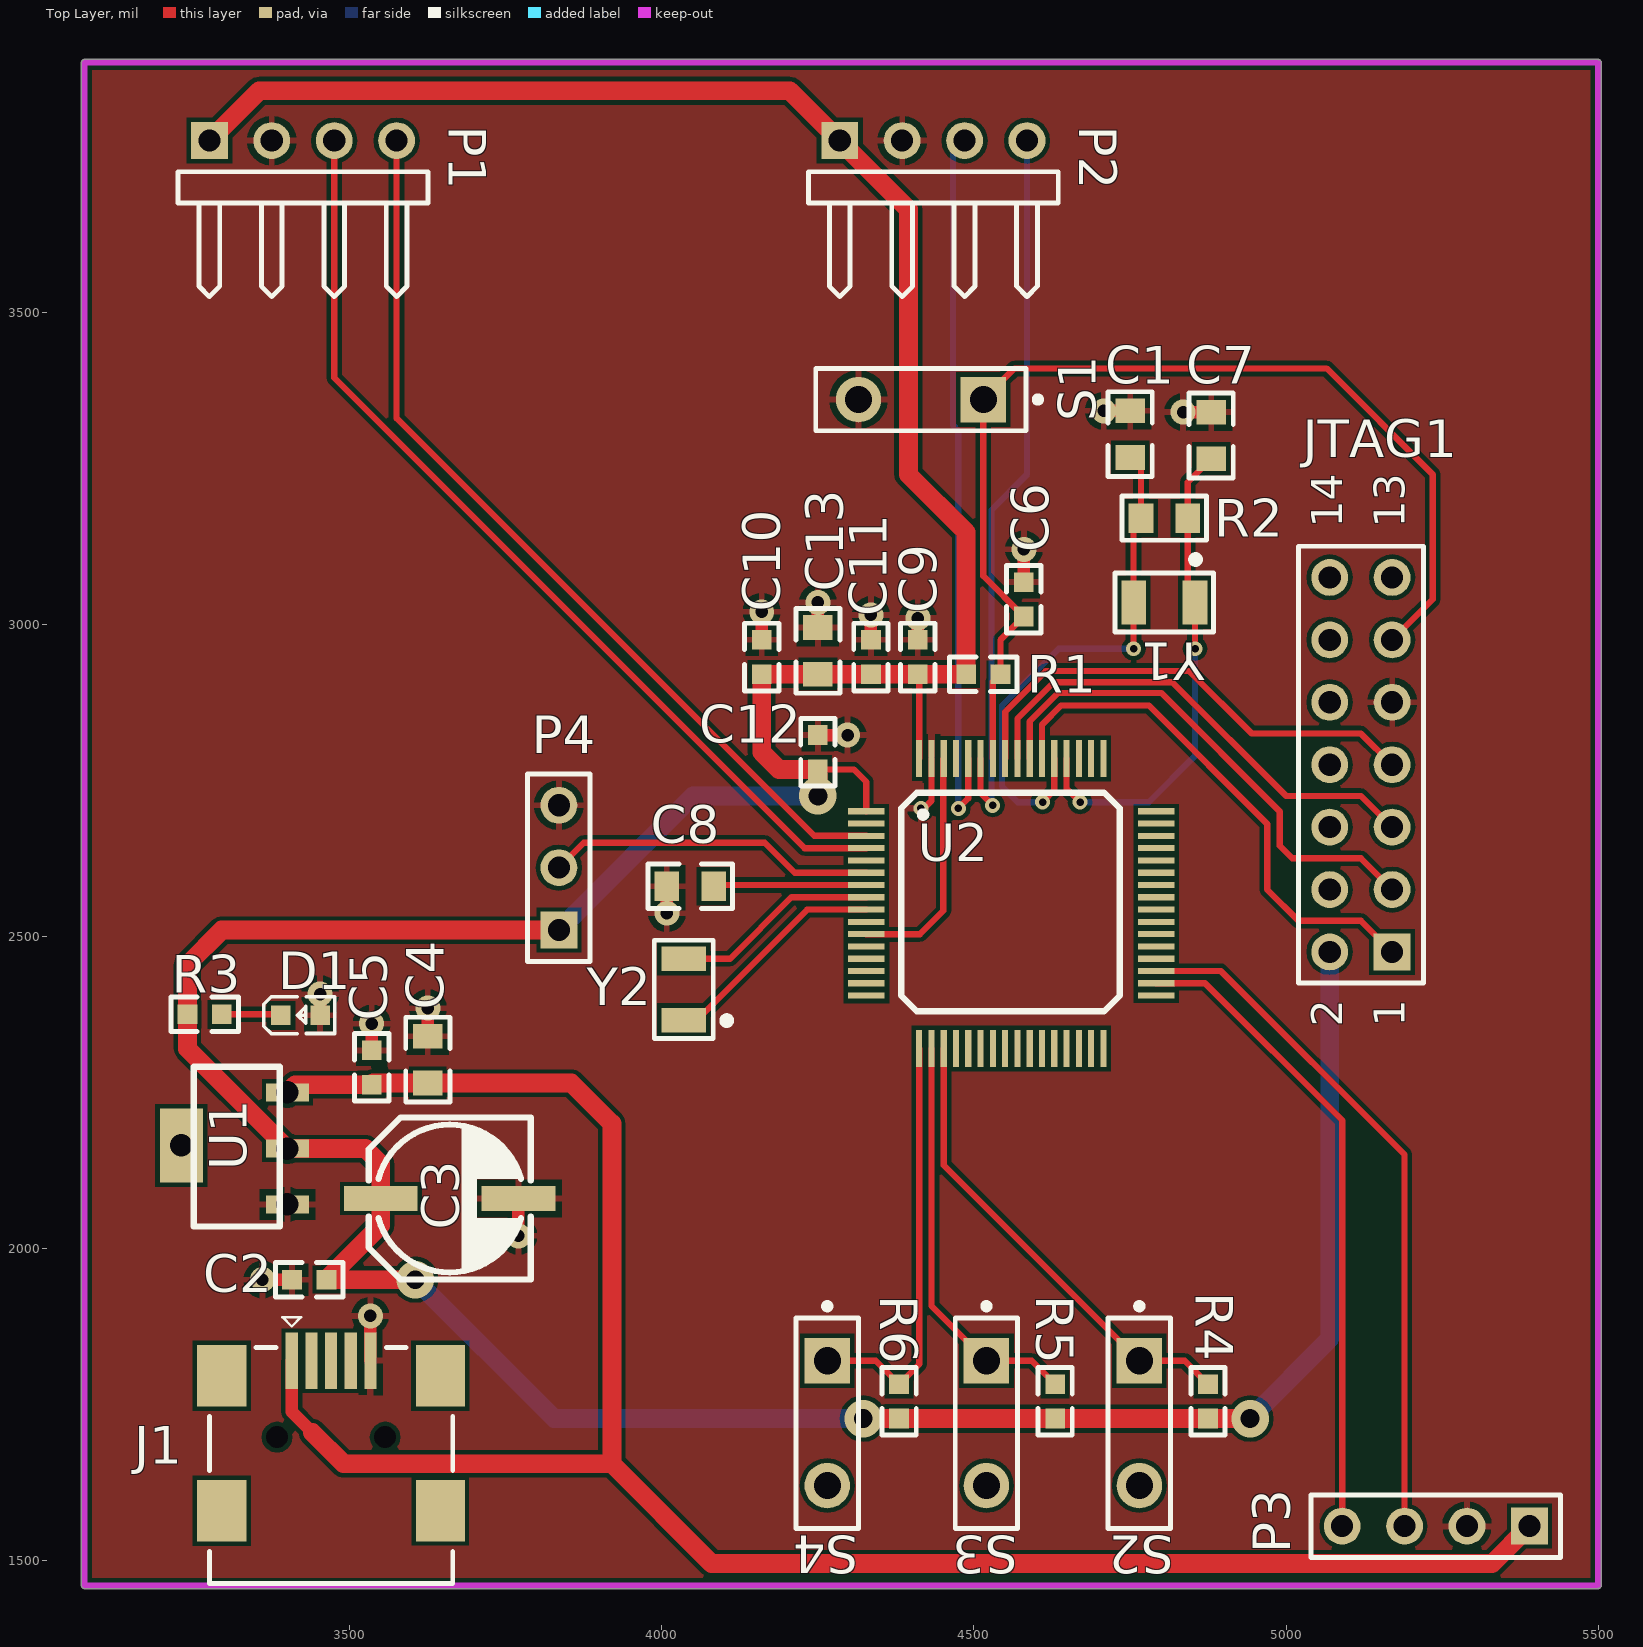
[diagram p0: Top Layer view]
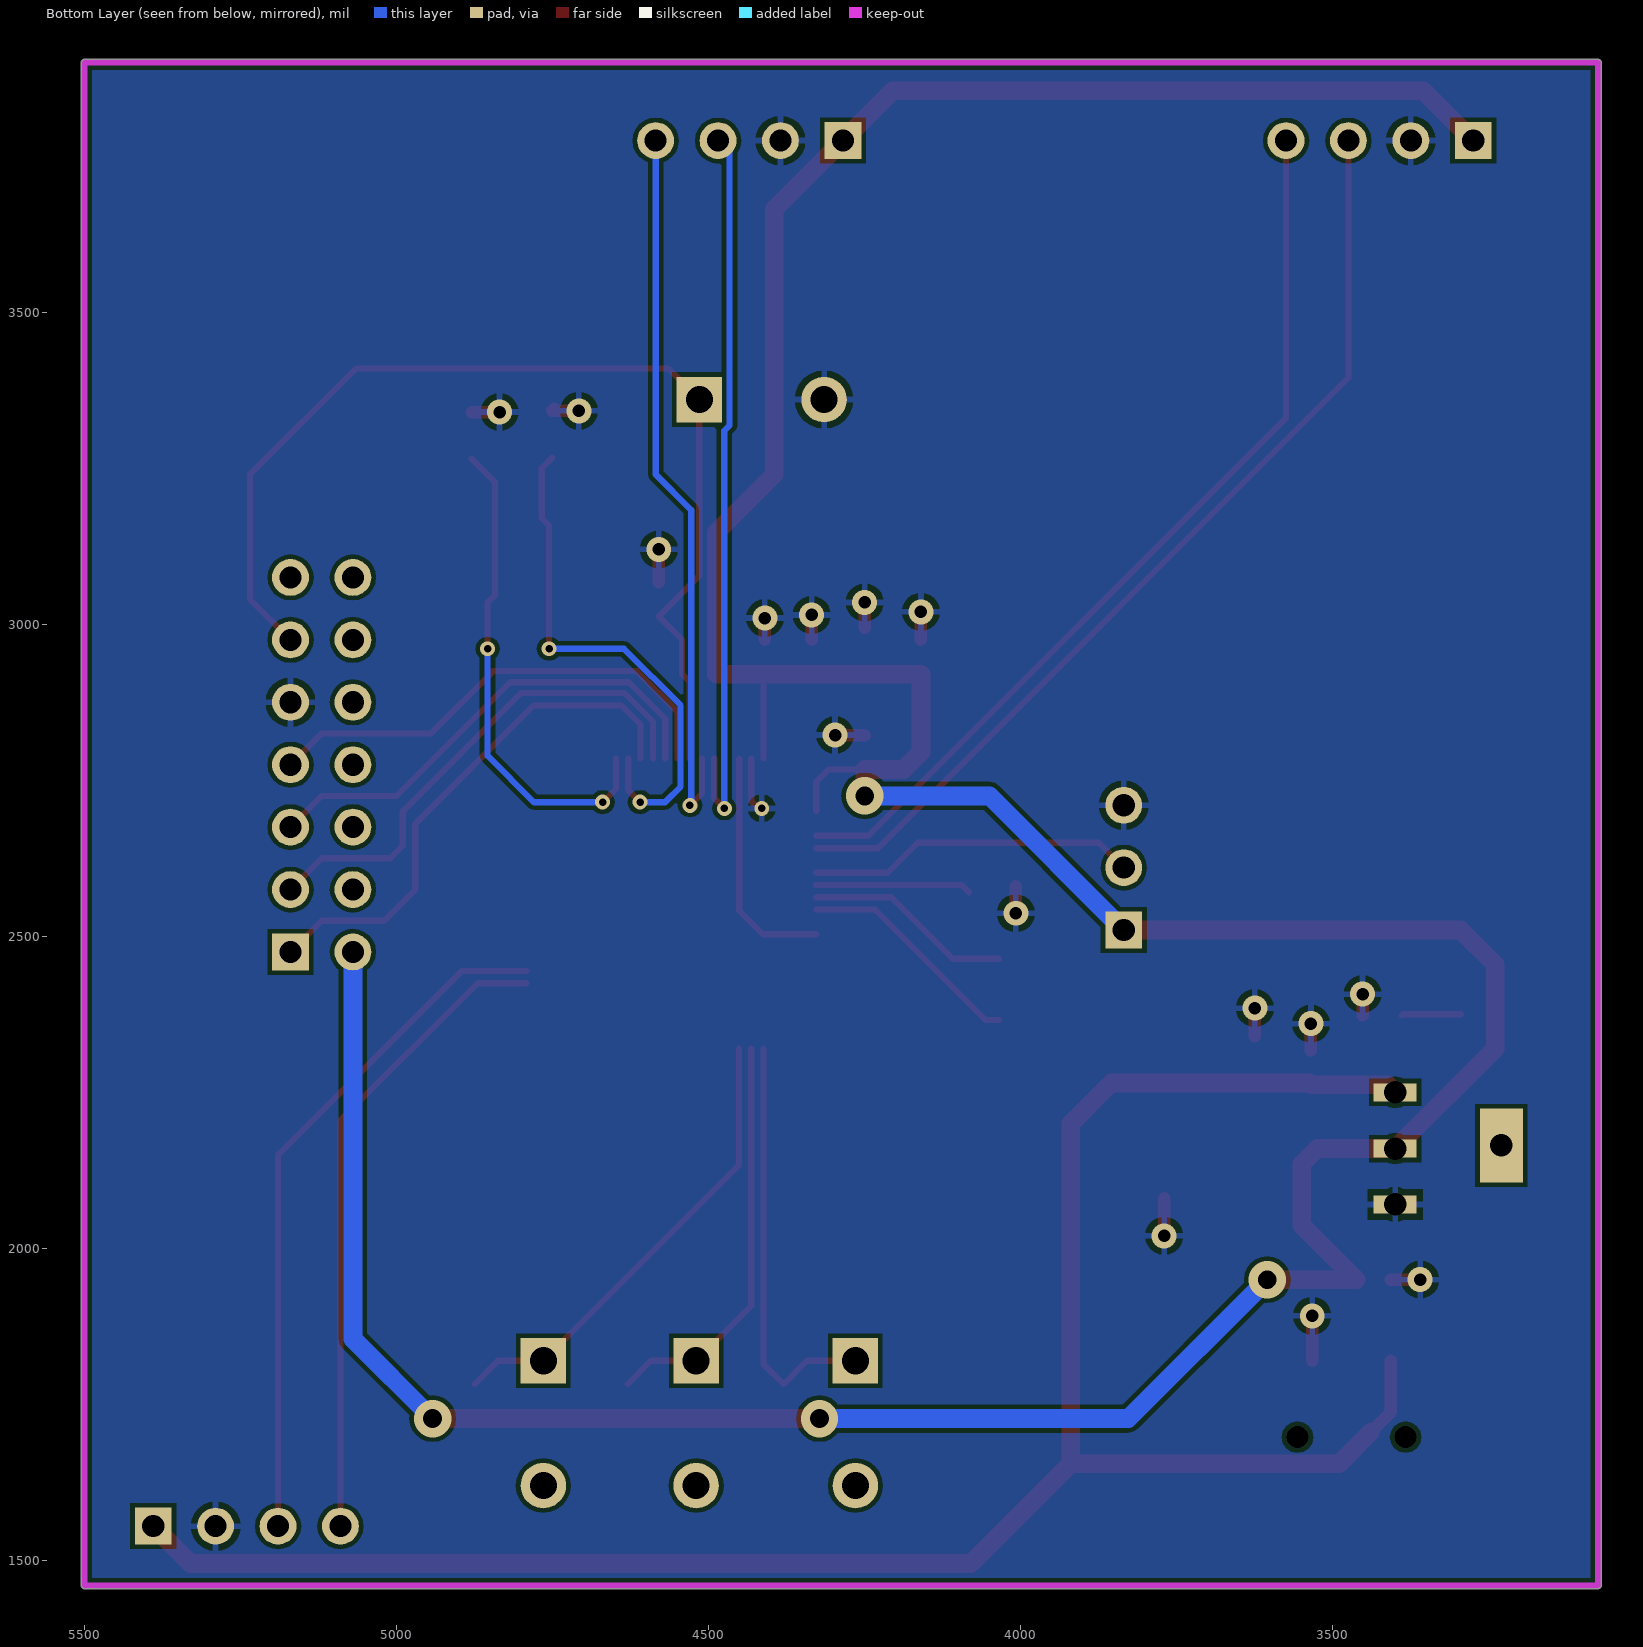
[diagram p1: Bottom Layer view, seen from below]
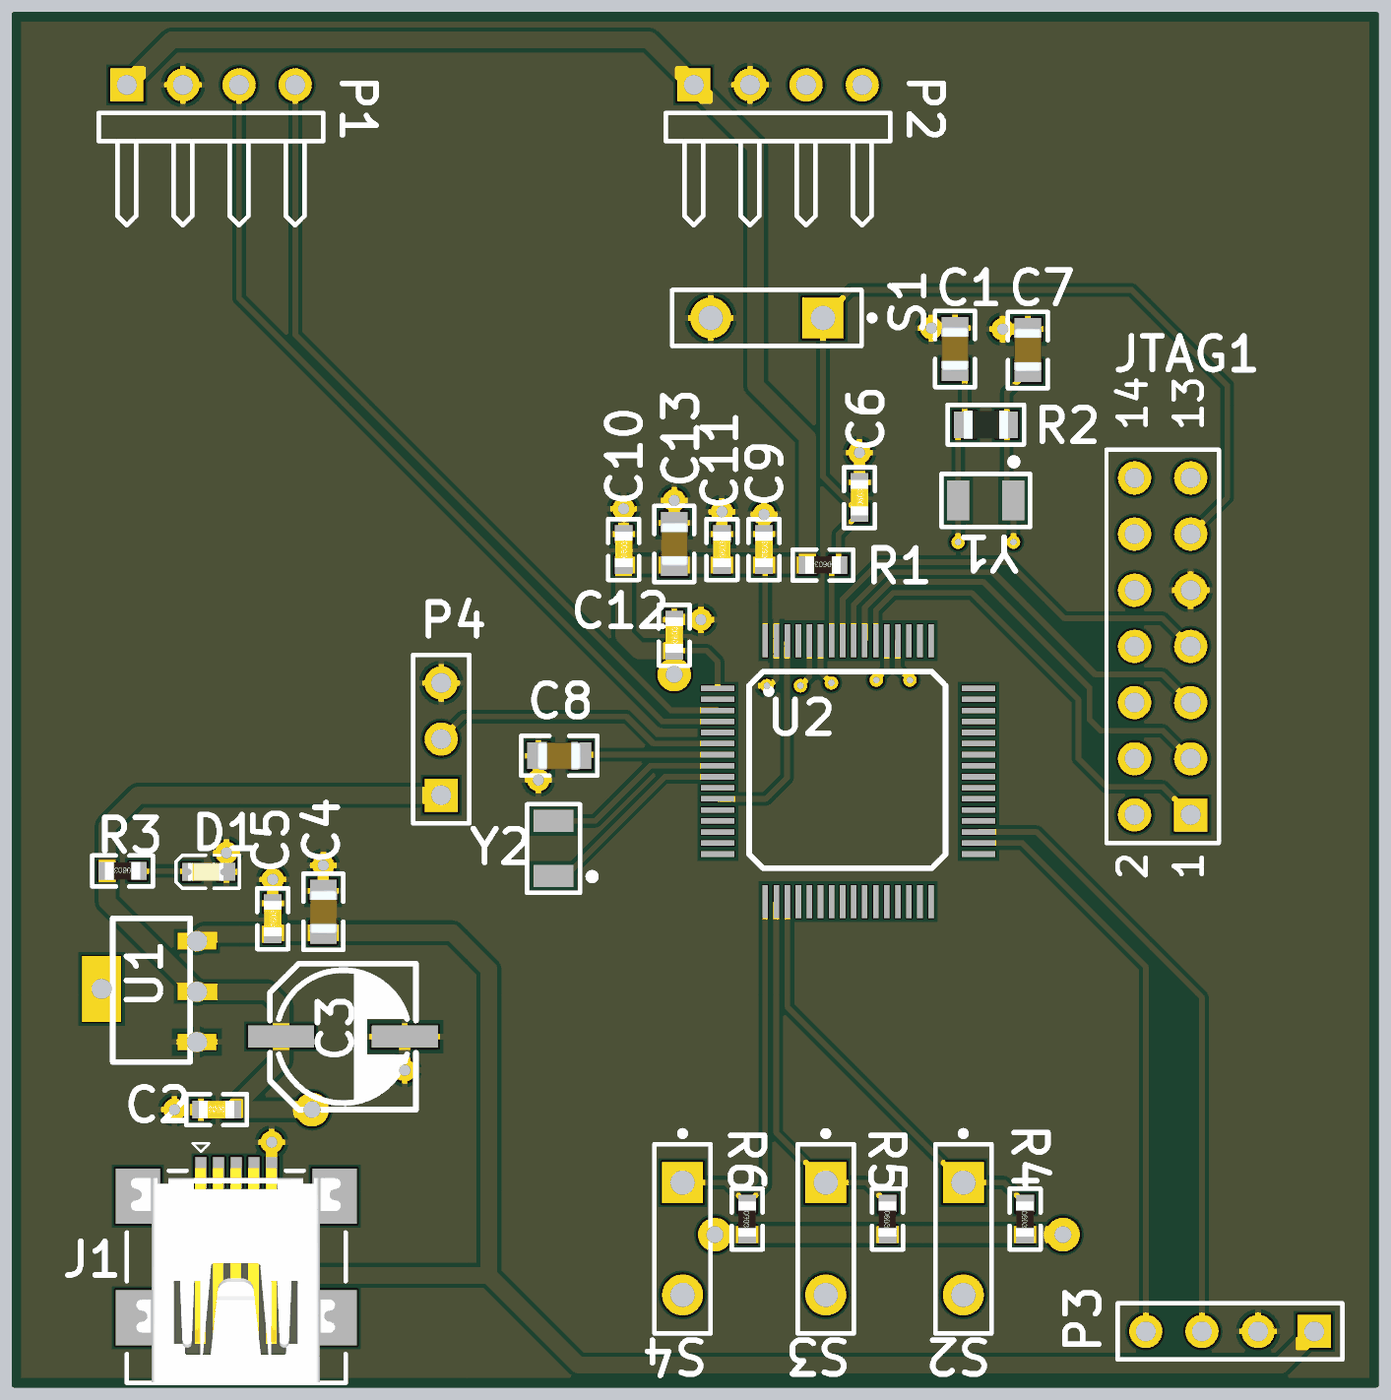
[diagram p2: 3D render of the assembled board from above, using the file's embedded part models]
# Altium PCB MISC82806.PcbDoc
Units mil, origin at the board's own origin, x right, y up, seen from the top; angles counter-clockwise.
Board outline 2435.03 x 2450.03 mil, 2 copper layers (Top Layer, Bottom Layer); 34 components, 63 nets, 160 pads, 26 vias.

## Layer stack, top to bottom (the 12.6 mil dielectric is the usual default, probably not edited)
Top Solder: solder mask 0.4, Solder Resist, Dk 3.5
Top Layer: signal copper 1.4
Dielectric 1: dielectric 12.6, FR-4, Dk 4.8
Bottom Layer: signal copper 1.4
Bottom Solder: solder mask 0.4, Solder Resist, Dk 3.5

## Board outline
3069.99,1460 ccw(c3075,1460) 3075,1454.98 5500,1454.98 ccw(c5500,1460) 5505.02,1460 5505.02,3900 ccw(c5500,3900) 5500,3905.01 3075,3905.01 ccw(c3075,3900) 3069.99,3900

## Design rules (kind name [scope] priority, off if disabled: settings)
Clearance [All] p1: gap=7
MinimumSolderMaskSliver [All] p1: minsoldermaskwidth=0
PolygonConnect [All] p1: connectstyle=Relief reliefconductorwidth=10 reliefentries=4 polygonreliefangle="90 Angle" airgapwidth=10
RoutingVias [All] p1: holewidth=28 width=50 viastyle="Through Hole" minholewidth=28 minwidth=50 maxholewidth=28 maxwidth=50
SilkToSilkClearance [All] p1: silktosilkclearance=0
SilkToSolderMaskClearance [IsPad] p1: minsilkscreentomaskgap=0 clearancetoexposedcopper=TRUE
SolderMaskExpansion [All] p1: expansion=4
Width [All] p1: maxlimit=30 minlimit=10 preferedwidth=10
27 further rules are at their usual default settings.

## Components (designator, comment, footprint, x,y, rotation, side; value= is the part's Value field where it differs from the comment)
C1 "S0805-20P" 0805C 4750,3305 r270 top
C2 "104" 0603C 3435,1950 r180 top
C3 "10uF" 贴片电容 3660,2080 r270 top
C4 "10uF" 0805C 3625.28,2302.01 r90 top
C5 "104" 0603C 3535,2290 r90 top
C6 "104" 0603C 4580,3040 r90 top
C7 "S0805-20P" 0805C 4879.72,3302.99 r270 top
C8 "S0805-20P" 0805C 4045,2580 r0 top
C9 "104" 0603C 4410,2947.56 r90 top
C10 "104" 0603C 4160,2947.56 r90 top
C11 "104" 0603C 4335,2947.56 r90 top
C12 "104" 0603C 4250,2795 r90 top
C13 "106" 0805C 4250.28,2957.01 r90 top
D1 "LED0" LED0603-RD 3420.93,2373.5 r0 top
J1 "Mini-USB" USB-MINI-A 3407.01,1820 r0 top
JTAG1 "DIP14" HDR2X7 5170,2475 r90 top
P1 "OLED" HDR1X4H 3275,3775 r0 top
P2 "BMP108" HDR1X4H 4285,3775 r0 top
P3 "Bluetooth module" HDR1X4 5390,1555 r180 top
P4 "Buzzer" HDR1X3 3835,2510 r90 top
R1 "10K" 0603R 4515,2920 r180 top
R2 "RC-1M" 0805R 4805,3170 r180 top
R3 "510R" 0603R 3267.44,2375 r180 top
R4 "10K" 0603R 4875,1755 r270 top
R5 "10K" 0603R 4630,1755 r270 top
R6 "10K" 0603R 4380,1755 r270 top
S1 "SW-SPST" SPST-2 4415,3360 r180 top
S2 "SW-PB" SPST-2 4765,1720 r270 top
S3 "SW-PB" SPST-2 4520,1720 r270 top
S4 "SW-PB" SPST-2 4265,1720 r270 top
U1 "AMS1117-3.3" AMS1117-3.3 3289.72,2052.95 r90 top
U2 "MSP430F149" MSP430F149 4559.84,2552.72 r0 top
Y1 "8M" XTAL-SMD-NX3215SA-32.768K-STD-MUS-2 4805,3035 r180 top
Y2 "32768" XTAL-SMD-NX3215SA-32.768K-STD-MUS-2 4035,2415 r90 top

## Footprints (in the part's own frame and the unit in brackets; to place one, negate y for a bottom-side part, rotate by r counter-clockwise, add the part's x,y. Pads: shape width x height; smd on the part's side, far side on the other; paste and mask are expansions set on the pad)
0603C [mm]
  rect 0.8x0.8 smd: 1(-0.7,0) 2(0.7,0)
  silkscreen extent -1.38,-0.7 1.38,0.7, body extent -0.8,-0.4 0.8,0.4, height 0.8
0603R [mm]
  rect 0.8x0.8 smd: 1(-0.7,0) 2(0.7,0)
  silkscreen extent -1.38,-0.7 1.38,0.7, body extent -0.8,-0.41 0.8,0.39, height 0.8
0805C [mm]
  rect 1x1.2 smd: 1(-0.94,0.007) 2(0.96,0.007)
  silkscreen extent -1.72,-0.89 1.74,0.91, body extent -1,-0.63 1,0.63, height 1.45
0805R [mm]
  rect 1x1.2 smd: 1(-0.95,0) 2(0.95,0)
  silkscreen extent -1.73,-0.9 1.73,0.9, body extent -1,-0.64 1,0.64, height 0.65
AMS1117-3.3 [mm]
  rect 0.74x1.75 hole 0.914 paste+0 mask+0.051: 1(0.444,-2.801) 2(2.719,-2.801) 3(5.005,-2.801)
  rect 3x1.75 hole 0.914 paste+0 mask+0.051: 4(2.846,1.517)
  silkscreen extent -0.46,-2.49 6.04,1.01
HDR1X3 [mm] "Connector; Header; 3 Position"
  rect 1.5x1.5 hole 0.9: 1(0,0)
  round 1.5 hole 0.9: 2(2.54,0) 3(5.08,0)
  silkscreen extent -1.27,-1.27 6.35,1.27
HDR1X4 [mm] "Connector; Header; 4 Position"
  rect 1.5x1.5 hole 0.9: 1(0,0)
  round 1.5 hole 0.9: 2(2.54,0) 3(5.08,0) 4(7.62,0)
  silkscreen extent -1.27,-1.27 8.89,1.27
HDR1X4H [mm] "Connector; Header; 4 Position; Right Angle"
  rect 1.5x1.5 hole 0.9: 1(0,0)
  round 1.5 hole 0.9: 2(2.54,0) 3(5.08,0) 4(7.62,0)
  silkscreen extent -1.27,-6.35 8.89,-1.27
HDR2X7 [mm] "Connector; Header; 7x2 Position"
  rect 1.5x1.5 hole 0.9: 1(0,0)
  round 1.5 hole 0.9: 2(0,2.54) 3(2.54,0) 4(2.54,2.54) 5(5.08,0) 6(5.08,2.54) 7(7.62,0) 8(7.62,2.54) 9(10.16,0) 10(10.16,2.54) 11(12.7,0) 12(12.7,2.54) 13(15.24,0) 14(15.24,2.54)
  silkscreen extent -1.27,-1.27 16.51,3.81
LED0603-RD [mm]
  rect 0.8x0.8 smd: 1(-0.8,-0.003) 2(0.8,0.003)
  silkscreen extent -1.49,-0.75 1.39,0.76, body extent -0.93,-0.4 0.67,0.4, height 0.55
MSP430F149 [mm]
  rect 1.5x0.25 smd paste+0 mask+0.051: 1(-5.9,3.75) 2(-5.9,3.25) 3(-5.9,2.75) 4(-5.9,2.25) 5(-5.9,1.75) 6(-5.9,1.25) 7(-5.9,0.75) 8(-5.9,0.25) 9(-5.9,-0.25) 10(-5.9,-0.75) 11(-5.9,-1.25) 12(-5.9,-1.75) 13(-5.9,-2.25) 14(-5.9,-2.75) 15(-5.9,-3.25) 16(-5.9,-3.75) 33(5.9,-3.75) 34(5.9,-3.25) 35(5.9,-2.75) 36(5.9,-2.25) 37(5.9,-1.75) 38(5.9,-1.25) 39(5.9,-0.75) 40(5.9,-0.25) 41(5.9,0.25) 42(5.9,0.75) 43(5.9,1.25) 44(5.9,1.75) 45(5.9,2.25) 46(5.9,2.75) 47(5.9,3.25) 48(5.9,3.75)
  rect 0.25x1.5 smd paste+0 mask+0.051: 17(-3.75,-5.9) 18(-3.25,-5.9) 19(-2.75,-5.9) 20(-2.25,-5.9) 21(-1.75,-5.9) 22(-1.25,-5.9) 23(-0.75,-5.9) 24(-0.25,-5.9) 25(0.25,-5.9) 26(0.75,-5.9) 27(1.25,-5.9) 28(1.75,-5.9) 29(2.25,-5.9) 30(2.75,-5.9) 31(3.25,-5.9) 32(3.75,-5.9) 49(3.75,5.9) 50(3.25,5.9) 51(2.75,5.9) 52(2.25,5.9) 53(1.75,5.9) 54(1.25,5.9) 55(0.75,5.9) 56(0.25,5.9) 57(-0.25,5.9) 58(-0.75,5.9) 59(-1.25,5.9) 60(-1.75,5.9) 61(-2.25,5.9) 62(-2.75,5.9) 63(-3.25,5.9) 64(-3.75,5.9)
  silkscreen extent -4.48,-4.38 4.41,4.51
SPST-2 [mm] "Switch; 2 Leads"
  rect 1.85x1.85 hole 1.1: 1(-2.54,0)
  round 1.85 hole 1.1: 2(2.54,0)
  silkscreen extent -4.89,-1.27 4.28,1.27
USB-MINI-A [mm]
  rect 2x2.5 smd: 0(-2.85,-6.108) 0(-2.85,-0.608) 0(6.05,-6.108) 0(6.05,-0.608)
  rect 0.5x2.3 smd: 1(0,0) 2(0.8,0) 3(1.6,0) 4(2.4,0) 5(3.2,0)
  round 0.6 hole 0.9 unplated: MH1(3.8,-3.108) MH2(-0.6,-3.108)
  silkscreen extent -3.35,-9.06 6.55,1.78, body extent -3.17,-9.04 6.33,0.66, height 3.95
XTAL-SMD-NX3215SA-32.768K-STD-MUS-2 [mm] "Crystal; 3.2mm W X 1.5mm L X 0.9mm H body"
  rect 1x1.8 smd paste+0 mask+0: 1(-1.25,0) 2(1.25,0)
  silkscreen extent -2,-1.9 2,1.2, body extent -1.6,-0.75 1.6,0.75, height 0.9
贴片电容 [mm]
  rect 1x3 smd paste+0 mask+0.102: 1(0,-2.8) 2(0,2.8)
  silkscreen extent -3.3,-3.3 3.3,3.3

## Part data
C1 C2 C7 C8: library part Cap, "Capacitor"
C3: library part "CAPACITOR POL", "Capacitor"
C4: library part ELECTRO2
C5: library part CAP, "Capacitor"
C6 C9 C10 C11 C12 C13: library part CAP1, "Capacitor"
D1: "Typical INFRARED GaAs LED"
J1: library part "Header 5", "Header, 5-Pin"
JTAG1: "Connectors"
P1 P2: library part "Header 4H", "Header, 4-Pin, Right Angle"
P3: library part "Header 4", "Header, 4-Pin"
P4: library part "Header 3", "Header, 3-Pin"
R1 R3 R4 R5 R6: library part R
R2: library part Res2, "Resistor"
S1: "Single-Pole, Single-Throw Switch"
S2 S3 S4: "Switch"
U1: library part LT1085CM-3.3
U2: "MCU"
Y1 Y2: library part XTAL, "Crystal Oscillator"

## Via types
v1: diameter 40, hole 20, Top Layer to Bottom Layer, 15 vias
v2: diameter 24, hole 12, Top Layer to Bottom Layer, 7 vias
v3: diameter 60, hole 30, Top Layer to Bottom Layer, 4 vias

## Nets (pads, with @x,y where several pads share a name; then routed paths per layer and width w, separated by ;. In a path a pad name is that pad's centre, name@x,y a point inside that pad or via, vN(x,y) a via of type N, cw(c..) or ccw(c..) an arc to the next point about the centre after c; other vN are vias at no path point)
3V3: C2.1 C3.1 C9.1 C10.1 C11.1 C12.1 C13.1 JTAG1.2 P1.1 P2.1 P4.1 R1.2 R3.2 R4.2 R5.2 R6.2 U1.2 U2.1 U2.64 | length 7117.3
  Top Layer w10: C12.1 4307.56,2767.44 4327.55,2747.45 U2.1 ; C9.1 4412.2,2917.8 U2.64
  Top Layer w30: P1.1 3355,3855 4205,3855 P2.1 4395,3665 4395,3240 4487.44,3147.56 R1.2 C9.1 C11.1 C13.1 C10.1 4160,2795 4187.56,2767.44 C12.1 v3(4250,2725) ; v3(3605,1950) C2.1 3549.76,2037.2 C3.1 3549.76,2135.24 3525,2160 U1.2 3239.88,2320.12 R3.2 3239.88,2454.88 3295,2510 P4.1 ; v3(4322.44,1727.44) R6.2 R5.2 R4.2 v3(4942.44,1727.44)
  Bottom Layer w30: v3(3605,1950) 3827.56,1727.44 v3(4322.44,1727.44) ; P4.1 4050,2725 v3(4250,2725) ; v3(4942.44,1727.44) 5070,1855 JTAG1.2
5V: C4.1 C5.1 J1.1 P3.1 U1.3 | length 3288.6
  Top Layer w20: J1.1 3407.01,1737.99 3440,1705
  Top Layer w30: U1.3 3412.44,2262.44 C5.1 3537.56,2265 C4.1 3855,2265 3920,2200 3920,1655 ; 3440,1705 3490,1655 3920,1655 ; P3.1 5330,1495 4080,1495 3920,1655
GND: C1.1 C2.2 C3.2 C4.2 C5.2 C6.2 C7.1 C8.1 C9.2 C10.2 C11.2 C12.2 C13.2 D1.2 J1.5 JTAG1.9 P1.2 P2.2 P3.2 P4.3 S1.2 U1.1 U2.63 | length 785.2
  Top Layer w10: v2(4415,2705) 4420,2705 4431.89,2716.89 U2.63
  Top Layer w20: v1(3360,1950) C2.2 ; D1.2 v1(3452.4,2407.4) ; J1.5 v1(3532.99,1892.01) ; C5.2 v1(3535,2360) ; C4.2 v1(3625,2385) ; v1(3770.24,2020.24) C3.2 ; v1(4007.99,2537.01) C8.1 ; C10.2 v1(4160,3020) ; C12.2 v1(4297.56,2822.56) ; C13.2 v1(4250,3035) ; C11.2 v1(4335,3015) ; C9.2 v1(4410,3010) ; C6.2 v1(4580,3120) ; v1(4707.99,3342.01) C1.1 C1.1@4747.28,3345 ; v1(4835,3340) C7.1
GNDA: U2.11 U2.62 | length 383.2
  Top Layer w10: U2.11 4413.51,2503.51 4451,2541 4451,2784.43 U2.62
NetC8_2: C8.2 U2.7 | length 249.7
  Top Layer w10: C8.2@4082.8,2570.28 4094.77,2582.25 U2.7
NetD1_1: D1.1 R3.1 | length 95.1
  Top Layer w10: R3.1 3387.82,2375 D1.1
NETLABEL41: U2.49
NetU2_8: U2.8 Y2.2 | length 333.3
  Top Layer w10: Y2.2 4109.21,2464.21 4207.56,2562.56 U2.8
NetU2_9: U2.9 Y2.1 | length 365.9
  Top Layer w10: Y2.1 4055.79,2365.79 4232.88,2542.88 U2.9
P1.0: U2.12
P1.1: U2.13
P1.2: U2.14
P1.3: U2.15
P1.4: U2.16
P1.5: R6.1 S4.1 U2.17 | length 681.7
  Top Layer w10: S4.1 4342.56,1820 R6.1 4412.2,1814.76 U2.17
P1.6: R5.1 S3.1 U2.18 | length 662.4
  Top Layer w10: U2.18 4431.89,1908.11 S3.1 4592.56,1820 R5.1
P1.7: R4.1 S2.1 U2.19 | length 755.8
  Top Layer w10: U2.19 4451.57,2133.43 S2.1 4837.56,1820 R4.1
P2.0: U2.20
P2.1: U2.21
P2.2: U2.22
P2.3: U2.23
P2.4: U2.24
P2.5: U2.25
P2.6: U2.26
P2.7: U2.27
P3.0: U2.28
P3.1: U2.29
P3.2: U2.30
P3.3: U2.31
P3.4: U2.32
P3.5: U2.33
P3.6: P3.4 U2.34 | length 1038.9
  Top Layer w10: U2.34 4870.24,2424.76 5090,2205 P3.4
P3.7: P3.3 U2.35 | length 1114.8
  Top Layer w10: U2.35 4895.55,2444.45 5190,2150 P3.3
P4.0: U2.36
P4.1: U2.37
P4.2: U2.38
P4.3: U2.39
P4.4: U2.40
P4.5: U2.41
P4.6: U2.42
P4.7: U2.43
P5.0: U2.44
P5.1: U2.45
P5.2: U2.46
P5.3: U2.47
P5.4: U2.48
P5.7: U2.51
P6.0: P2.4 U2.59 | length 1172.5
  Top Layer w10: U2.59 4510.63,2729.37 v2(4530,2710)
  Bottom Layer w10: v2(4530,2710) 4528,2712 4528,3183 4585,3240 P2.4
P6.1: P2.3 U2.60 | length 1167.7
  Top Layer w10: v2(4475,2705) 4490.94,2720.94 U2.60
  Bottom Layer w10: v2(4475,2705) 4475,3310.19 4466.58,3318.61 4466.58,3756.58 P2.3
P6.2: U2.61
P6.3: U2.2
P6.4: P1.4 U2.3 | length 1474.7
  Top Layer w10: P1.4 3575,3330 4244.01,2660.99 U2.3
P6.5: P1.3 U2.4 | length 1544.7
  Top Layer w10: P1.3 3475,3395 4228.7,2641.3 U2.4
P6.6: U2.5
P6.7: P4.2 U2.6 | length 529
  Top Layer w10: P4.2 3875,2650 4165,2650 4213.07,2601.93 U2.6
RESET: C6.1 JTAG1.11 R1.1 S1.1 U2.58 | length 1725.6
  Top Layer w10: U2.58 4530.31,2907.75 R1.1 4542.56,2975 C6.1 4515,3077.44 S1.1 4565,3410 5065,3410 5235,3240 5235,3040 JTAG1.11
TCK: JTAG1.7 U2.57 | length 784.1
  Top Layer w10: U2.57 4550,2860 4615,2925 4845,2925 4945,2825 5120,2825 JTAG1.7
TDI: JTAG1.3 U2.55 | length 821.6
  Top Layer w10: U2.55 4589.37,2844.37 4635,2890 4800,2890 4990,2700 4990,2645 5010,2625 5120,2625 JTAG1.3
TDO: JTAG1.1 U2.54 | length 852.9
  Top Layer w10: U2.54 4609.05,2839.05 4640,2870 4780,2870 4970,2680 4970,2575 5020,2525 5120,2525 JTAG1.1
TMS: JTAG1.5 U2.56 | length 784.3
  Top Layer w10: U2.56 4569.68,2848.72 4627.96,2907 4818,2907 5000,2725 5120,2725 JTAG1.5
VEREF+: U2.10
XT2_IN: C1.2 R2.2 U2.53 Y1.2 | length 850
  Top Layer w10: v2(4610,2715) 4628.74,2733.74 U2.53 ; C1.2 4767.6,3249.88 R2.2 4755.79,3158.19 Y1.2 v2(4755.79,2960.79)
  Bottom Layer w10: v2(4610,2715) 4570,2715 4545,2740 4545,2870 4635.79,2960.79 v2(4755.79,2960.79)
XT2_OUT: C7.2 R2.1 U2.52 Y1.1 | length 790.3
  Top Layer w10: U2.52 4648.42,2736.58 v2(4670,2715) ; v2(4854.21,2960.79) Y1.1 4842.4,3046.81 R2.1 4842.4,3227.6 C7.2
  Bottom Layer w10: v2(4670,2715) 4780,2715 4854.21,2789.21 v2(4854.21,2960.79)
pads on no net: J1.0 J1.2 J1.3 J1.4 J1.MH1 J1.MH2 JTAG1.4 JTAG1.6 JTAG1.8 JTAG1.10 JTAG1.12 JTAG1.13 JTAG1.14 S2.2 S3.2 S4.2 U1.4 U2.50

## Polygon pours and split planes (outlines as drawn)
GND on Top Layer "G" (solid, remove dead copper, pour order 0): 2245,4060 2270,4085 5880,4085 5880,1645 5585,1350 5560,1325 2755,1325
GND on Bottom Layer "G" (solid, remove dead copper, pour order 2): 2970,3975 5525,3975 5535,3985 5585,3935 5585,1275 2995,1275 2970,1300

## Keep-outs
Keep-Out Layer:
  lines w10: 4545,3900 5500,3900 5500,1460 3075,1460 3075,3900 4700,3900